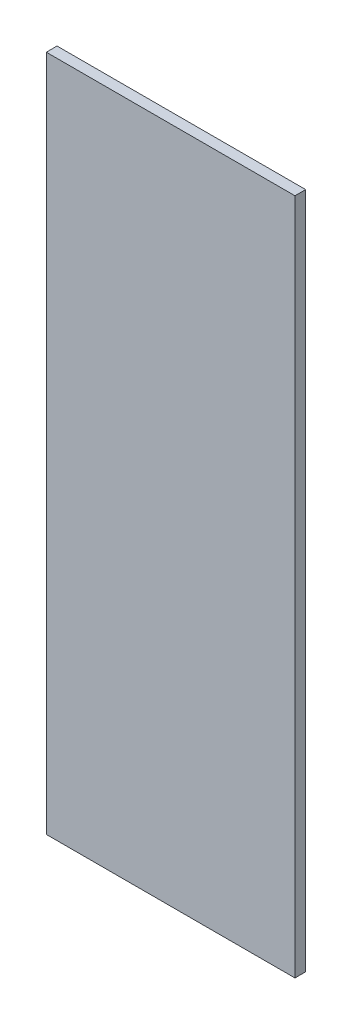
from build123d import *

# Parameters (mm, degrees)
SKETCH_1_W           = 820
SKETCH_1_H           = 1820
EXTRUDE_1_DEPTH      = 25
SKETCH_2_OUTSIDE_W   = 1221.27
SKETCH_2_OUTSIDE_H   = 2221.27
SKETCH_2_OUTSIDE_W_2 = 580
SKETCH_2_OUTSIDE_H_2 = 1580
CUT_EXTRUDE_1_DEPTH  = 999.411237918


with BuildPart() as part:
    # 草图1 → 凸台-拉伸1 (new body)
    with BuildSketch(Plane.XY):
        Rectangle(SKETCH_1_W, SKETCH_1_H)
    extrude(amount=EXTRUDE_1_DEPTH)

    # 草图2 outside → 切除-拉伸1 (cut, through all)
    with BuildSketch(Plane.XY.offset(25)):
        Rectangle(SKETCH_2_OUTSIDE_W, SKETCH_2_OUTSIDE_H)
        Rectangle(SKETCH_2_OUTSIDE_W_2, SKETCH_2_OUTSIDE_H_2, mode=Mode.SUBTRACT)
    extrude(amount=-CUT_EXTRUDE_1_DEPTH, mode=Mode.SUBTRACT)


solid = part.part
